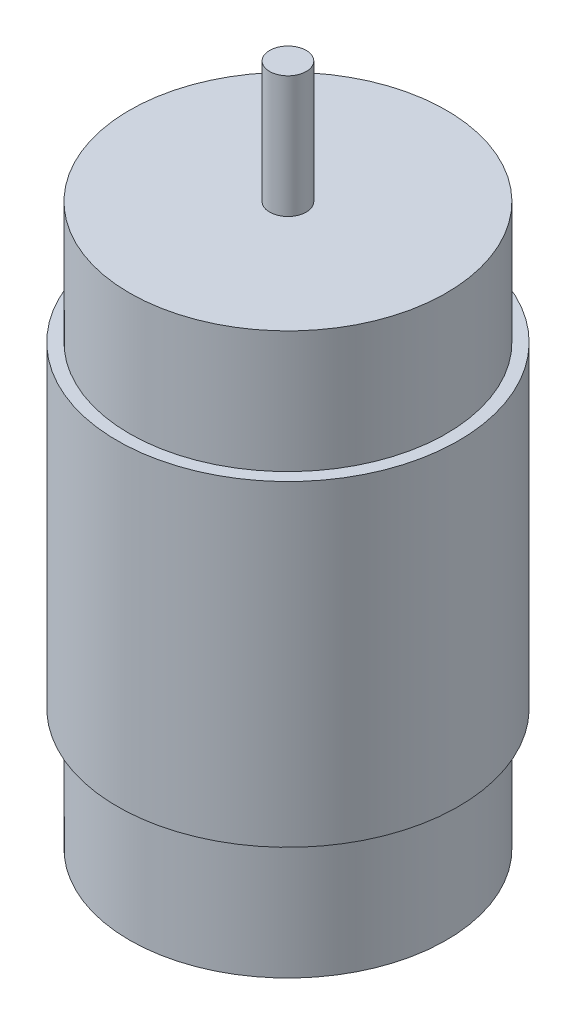
SolidWorks part; units mm, degrees
material "Медь"
ref_plane "Front" through (0, 0, 0) normal (0, 0, 1) x (1, 0, 0)
ref_plane "Top" through (0, 0, 0) normal (0, 1, 0) x (1, 0, 0)
ref_plane "Right" through (0, 0, 0) normal (1, 0, 0) x (0, 0, -1)
sketch "Sketch1" plane through (0, 0, 0) normal (0, 1, 0) x (1, 0, 0)
  circle A0 centre (0, 0) radius 13
  dimension "D1" = 26
extrude "Boss-Extrude1" add sketch "Sketch1" along normal blind 10
sketch "Sketch2" plane through (0, 10, 0) normal (0, 1, 0) x (1, 0, 0)
  circle A0 centre (0, 0) radius 14
  dimension "D1" = 28
extrude "Boss-Extrude2" add sketch "Sketch2" along normal blind 26
sketch "Sketch3" plane through (0, 36, 0) normal (0, 1, 0) x (1, 0, 0)
  circle A0 centre (0, 0) radius 13
  dimension "D1" = 26
extrude "Boss-Extrude3" add sketch "Sketch3" along normal blind 10
sketch "Sketch4" plane through (0, 46, 0) normal (0, 1, 0) x (1, 0, 0)
  circle A0 centre (0, 0) radius 1.5
  dimension "D1" = 3
extrude "Boss-Extrude4" add sketch "Sketch4" along normal blind 10
